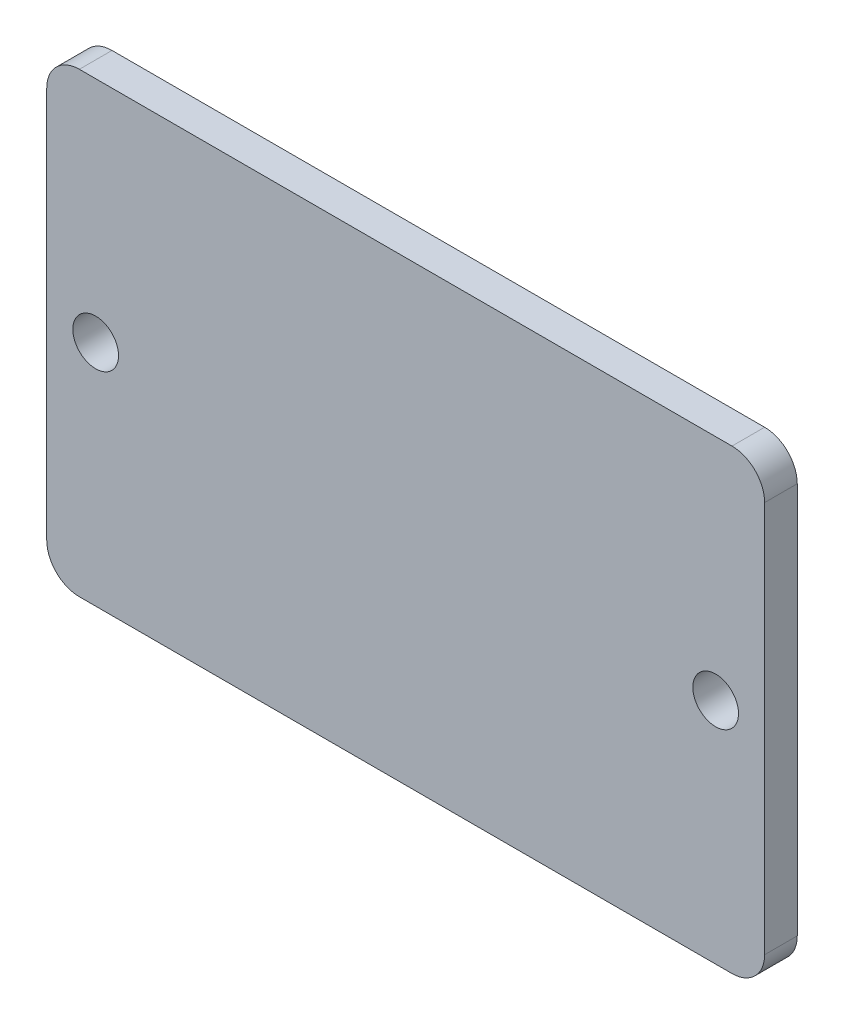
from build123d import *

# Parameters (mm, degrees)
SKETCH1_W           = 220
SKETCH1_H           = 140
SKETCH1_R           = 7
BOSS_EXTRUDE1_DEPTH = 10
FILLET1_R           = 10


with BuildPart() as part:
    # Sketch1 → Boss-Extrude1 (new body)
    with BuildSketch(Plane.XY):
        Rectangle(SKETCH1_W, SKETCH1_H)
        with Locations((-95, 0)):
            Circle(SKETCH1_R, mode=Mode.SUBTRACT)
        with Locations((95, 0)):
            Circle(SKETCH1_R, mode=Mode.SUBTRACT)
    extrude(amount=BOSS_EXTRUDE1_DEPTH)

    # Fillet1
    fillet1_edges = [part.edges().sort_by_distance(p)[0] for p in [
        (-110, 70, 5),
        (110, 70, 5),
        (110, -70, 5),
        (-110, -70, 5),
    ]]
    fillet(fillet1_edges, radius=FILLET1_R)


solid = part.part
